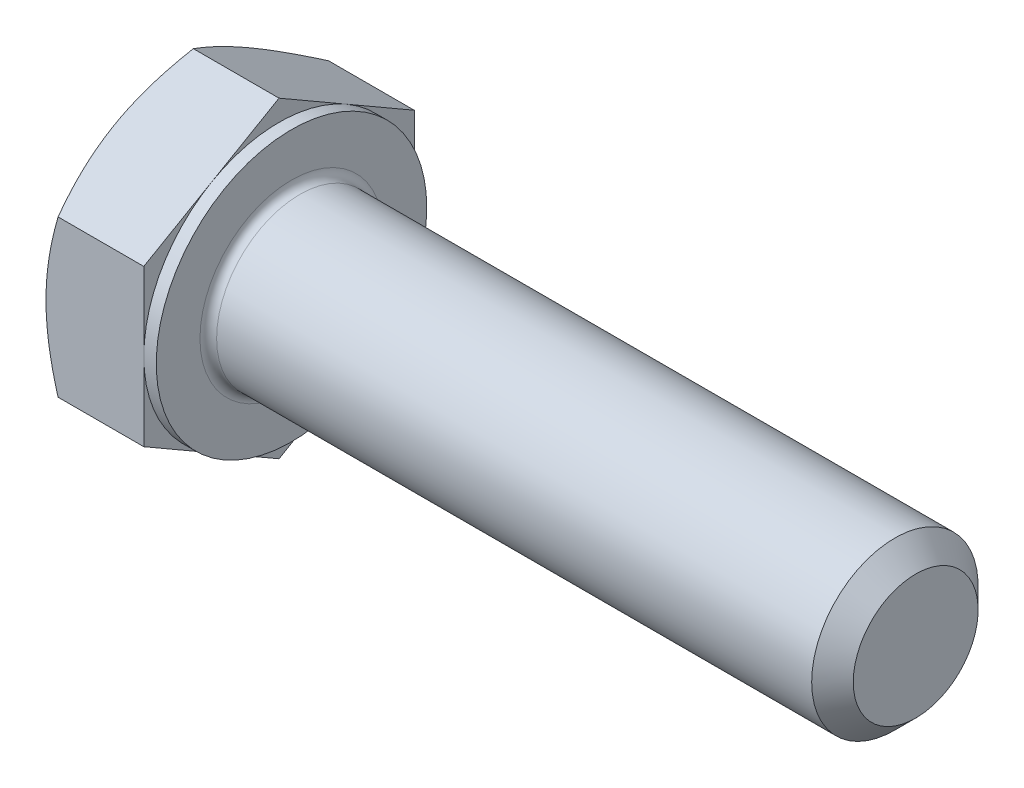
SolidWorks part; units mm, degrees
extrude "基体-拉伸" add sketch "草图1" along normal blind 5.3
sketch "草图1" plane through (0, 0, 0) normal (1, 0, 0) x (0, 0, -1)
  line L0 (6.5, 3.7528) -> (6.5, -3.7528)
  line L1 (-6.5, 3.7528) -> (-6.5, -3.7528)
  line L2 (6.5, -3.7528) -> (0, -7.5056)
  line L3 (0, -7.5056) -> (-6.5, -3.7528)
  line L4 (6.5, 3.7528) -> (0, 7.5056)
  line L5 (0, 7.5056) -> (-6.5, 3.7528)
revolve "切除-旋转1" cut sketch "草图3" angle 360 about L6
sketch "草图3" plane through (0, 0, 0) normal (0, 0, 1) x (1, 0, 0)
  line L0 (0, 6.5) -> (3.4673, 12.5056)
  line L1 (0, 7.5056) -> (0, 3.7528) construction
  line L2 (3.4673, 12.5056) -> (3.4673, 17.5056)
  line L3 (3.4673, 17.5056) -> (-10, 17.5056)
  line L4 (-10, 17.5056) -> (-10, 6.5)
  line L5 (-10, 6.5) -> (0, 6.5)
  line L6 (0, 0) -> (99.06, 0) construction
  line L7 (5.3, 7.5056) -> (0, 7.5056) construction
revolve "凸台-旋转1" add sketch "草图2" angle 360 about L7
sketch "草图2" plane through (0, 0, 0) normal (0, 0, 1) x (1, 0, 0)
  line L0 (0, 3.7528) -> (0, -3.7528) construction
  line L1 (0, 0) -> (35.3, 0)
  line L2 (0, 0) -> (0, 4)
  line L3 (0, 4) -> (35.3, 4)
  line L4 (35.3, 0) -> (35.3, 2.9175)
  line L5 (5.3, 7.5056) -> (5.3, 3.7528) construction
  line L7 (0, 0) -> (96.52, 0) construction
  line L8 (35.3, -2.9175) -> (90.335, -4) construction
  line L9 (0, -4) -> (90.335, -4) construction
  line L10 (6.55, 15.24) -> (6.55, -1.27) construction
  line L11 (5.3, 15.24) -> (5.3, -1.27) construction
  line L12 (5.3, 3.7528) -> (5.3, -3.7528) construction
  line L14 (35.3, 4) -> (35.3, 2.9175)
  dimension "l" = 30
  dimension "m" = 8
  dimension "Minor_dia" = 5.835
  dimension "p" = 1.25
  dimension "h" = 30
cosmetic thread "螺旋线1" parameters "Thread_length"=28.75, "Thread_minor"=5.835
material "3.6级"
ref_plane "前视" through (0, 0, 0) normal (0, 0, 1) x (1, 0, 0)
ref_plane "上视" through (0, 0, 0) normal (0, 1, 0) x (1, 0, 0)
ref_plane "右视" through (0, 0, 0) normal (1, 0, 0) x (0, 0, -1)
sketch "草图5" plane through (0, 0, 0) normal (0, 0, 1) x (1, 0, 0)
  line L0 (5.3, 6.5) -> (1.8327, 12.5056)
  line L1 (5.3, 7.5056) -> (5.3, 3.7528) construction
  line L2 (1.8327, 12.5056) -> (1.8327, 17.5056)
  line L3 (1.8327, 17.5056) -> (11.8327, 17.5056)
  line L4 (11.8327, 17.5056) -> (11.8327, 6.5)
  line L5 (11.8327, 6.5) -> (5.3, 6.5)
  line L7 (5.3, 7.5056) -> (0.5806, 7.5056) construction
  line L8 (0, 0) -> (99.06, 0) construction
  line L9 (0, 0) -> (99.06, 0) construction
revolve "切除-旋转2" cut sketch "草图5" angle 360 about L8
sketch "草图4" plane through (0, 0, 0) normal (0, 0, 1) x (1, 0, 0)
  line L1 (5.3, 7.5056) -> (5.3, 3.7528) construction
  line L2 (5.3, 6.5) -> (4.7, 6.5)
  line L3 (5.3, 6.5) -> (5.3, 17.5056)
  line L4 (5.3, 17.5056) -> (4.7, 17.5056)
  line L5 (0, 0) -> (95.25, 0) construction
  line L6 (0, 0) -> (96.52, 0) construction
  line L7 (4.7, 6.5) -> (4.7, 17.5056)
  line L8 (4.7194, 7.5056) -> (0.5806, 7.5056) construction
revolve "切除-旋转3" cut sketch "草图4" angle 360 about L5
chamfer "倒角" distance 1 angle 45 1 edges at (35.3, 0, 4)
fillet "圆角" radius 0.4 1 edges at (5.3, 0, -4)
sketch "草图6" plane through (0, 0, 0) normal (0, 0, 1) x (1, 0, 0)
  line L0 (6.325, -2.9175) -> (5.7, -4)
  line L1 (6.325, -2.9175) -> (6.95, -4)
  line L2 (6.95, -4) -> (6.95, -5)
  line L3 (-3.175, 0) -> (5.1513, 0) construction
  line L5 (6.95, -5) -> (5.7, -5)
  line L6 (5.7, -5) -> (5.7, -4)
  arc A0 (5.7, -4) -> (5.3, -4.4) centre (5.7, -4.4) ccw construction
revolve "切除-旋转4" [suppressed] cut sketch "草图6" angle 360 about L3
pattern_linear "阵列(线性)1" [suppressed]
equation "\"D3@草图1\" = \"s@草图1\" / 2"
equation "\"D4@草图1\" = \"D3@草图1\""
equation "\"D5@草图1\" = \"D4@草图1\""
equation "\"D1@草图3\" = \"s@草图1\" / 2"
equation "\"D1@草图5\" = \"s@草图1\" / 2"
equation "\"Head_ch_ang@草图5\" = \"Head_ch_ang@草图3\""
equation "\"D1@草图4\" = \"s@草图1\""
equation "\"Diameter@草图6\" = \"m@草图2\""
equation "\"Overcut@草图6\" = \"m@草图2\" * 1.25"
equation "\"Minor_dia@草图2\" = \"m@草图2\"-\"p@草图2\" * 1.732"
equation "\"Thread_minor@螺旋线1\" = \"Minor_dia@草图2\""
equation "\"Thread_minor@草图6\" = \"Minor_dia@草图2\""
equation "\"D1@倒角\" = \"p@草图2\"*0.8"
equation "\"Thread_length@螺旋线1\" = \"l@草图2\" - \"p@草图2\""
equation "\"Num_threads@阵列(线性)1\" = \"l@草图2\" / \"p@草图2\""
